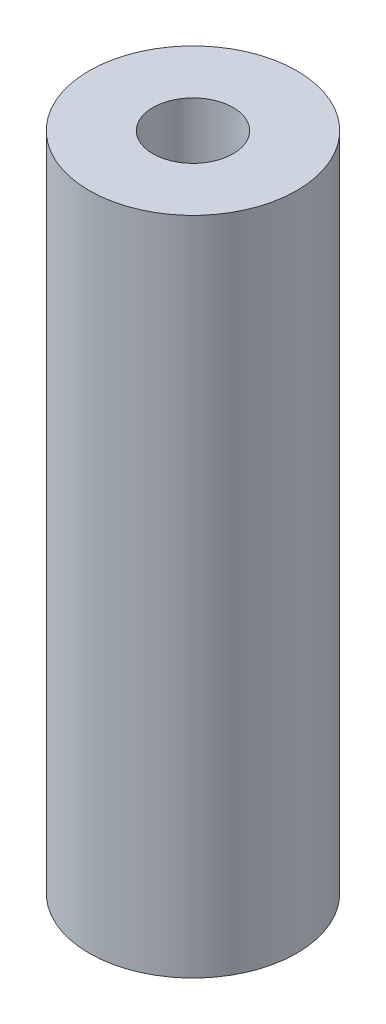
from build123d import *

# Parameters (mm, degrees)
SKETCH1_R              = 11
BOSS_EXTRUDE1_DEPTH    = 70
M10_TAPPED_HOLE1_D     = 8.5
M10_TAPPED_HOLE1_DEPTH = 25
M10_TAPPED_HOLE1_TIP   = 2.553657631


with BuildPart() as part:
    # Sketch1 → Boss-Extrude1 (new body)
    with BuildSketch(Plane(origin=(0, 0, 0), x_dir=(1, 0, 0), z_dir=(0, 1, 0))):
        with Locations(Location((0, 0, 0), (0, 0, 270))):
            Circle(SKETCH1_R)
    extrude(amount=BOSS_EXTRUDE1_DEPTH)

    # M10 Tapped Hole1
    with Locations(Plane(origin=(0, 70, 0), x_dir=(1, 0, 0), z_dir=(0, 1, 0))):
        with Locations((0, 0)):
            Hole(M10_TAPPED_HOLE1_D / 2, depth=M10_TAPPED_HOLE1_DEPTH)
            with Locations((0, 0, -(M10_TAPPED_HOLE1_DEPTH + M10_TAPPED_HOLE1_TIP / 2))):  # 118° drill point
                Cone(0, M10_TAPPED_HOLE1_D / 2, M10_TAPPED_HOLE1_TIP, mode=Mode.SUBTRACT)


solid = part.part
